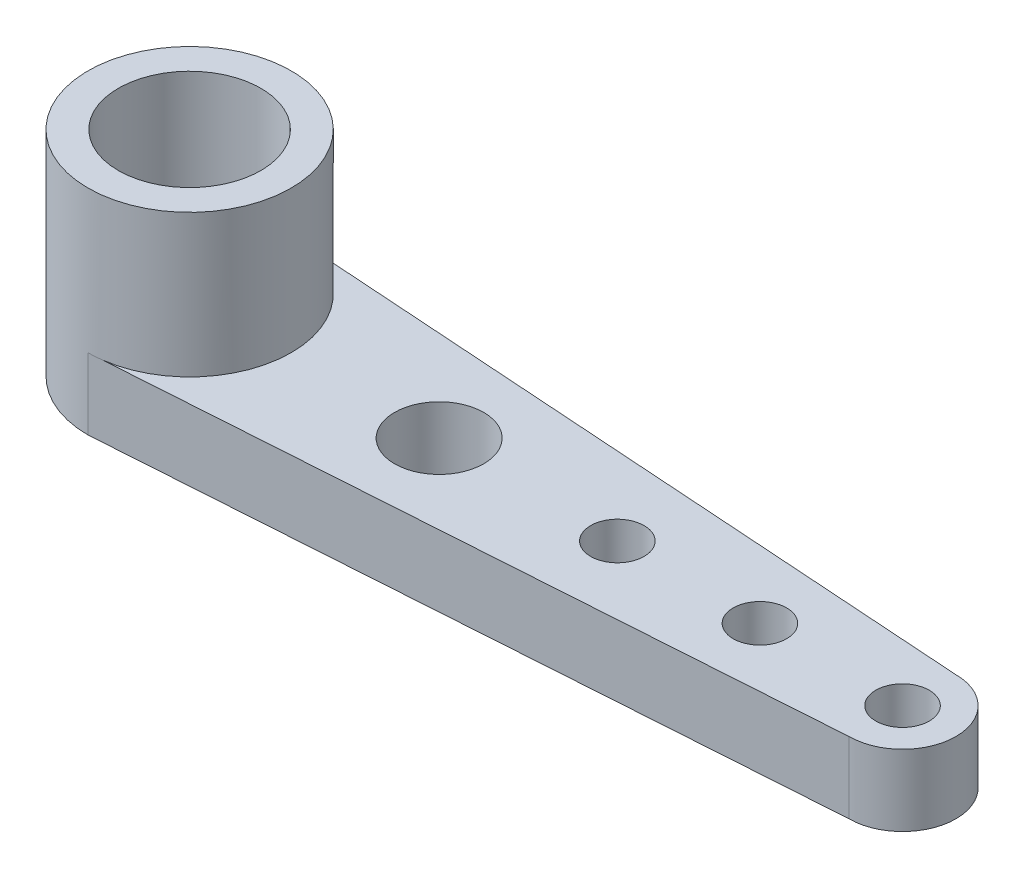
SolidWorks part; units mm, degrees
ref_plane "Front Plane" through (0, 0, 0) normal (0, 0, 1) x (1, 0, 0)
ref_plane "Top Plane" through (0, 0, 0) normal (0, 1, 0) x (1, 0, 0)
ref_plane "Right Plane" through (0, 0, 0) normal (1, 0, 0) x (0, 0, -1)
sketch "Sketch1" plane through (0, 0, 0) normal (0, 1, 0) x (1, 0, 0)
  line L1 (0, 2.8503) -> (20, 1.5)
  line L2 (0, -2.8503) -> (20, -1.5)
  arc A0 (0, 2.8503) -> (0, -2.8503) centre (0, 0) ccw
  arc A1 (20, -1.5) -> (20, 1.5) centre (20, 0) ccw
  dimension "D1" = 20
  dimension "D2" = 1.5
extrude "Boss-Extrude1" add sketch "Sketch1" along normal blind 2
sketch "Sketch2" plane through (0, 2, 0) normal (0, 1, 0) x (1, 0, 0)
  circle A0 centre (0, 0) radius 2.8503
  circle A1 centre (0, 0) radius 2
  dimension "D1" = 4
extrude "Boss-Extrude2" add sketch "Sketch2" along normal blind 4
sketch "Sketch3" plane through (0, 0, 0) normal (0, -1, 0) x (1, 0, 0)
  line L0 (15.25, 0) -> (12.75, 0) construction
  line L1 (11.25, 0) -> (8.25, 0) construction
  line L2 (5.75, 0) -> (0, 0) construction
  circle A0 centre (16, 0) radius 0.75
  circle A1 centre (12, 0) radius 0.75
  circle A2 centre (7, 0) radius 1.25
  circle A3 centre (20, 0) radius 0.75
  dimension "D4" = 1.5
  dimension "D5" = 1.5
  dimension "D6" = 2.5
  dimension "D7" = 1.5
  dimension "D1" = 4
  dimension "D2" = 4
  dimension "D3" = 5
extrude "Cut-Extrude1" cut sketch "Sketch3" against normal blind 10
